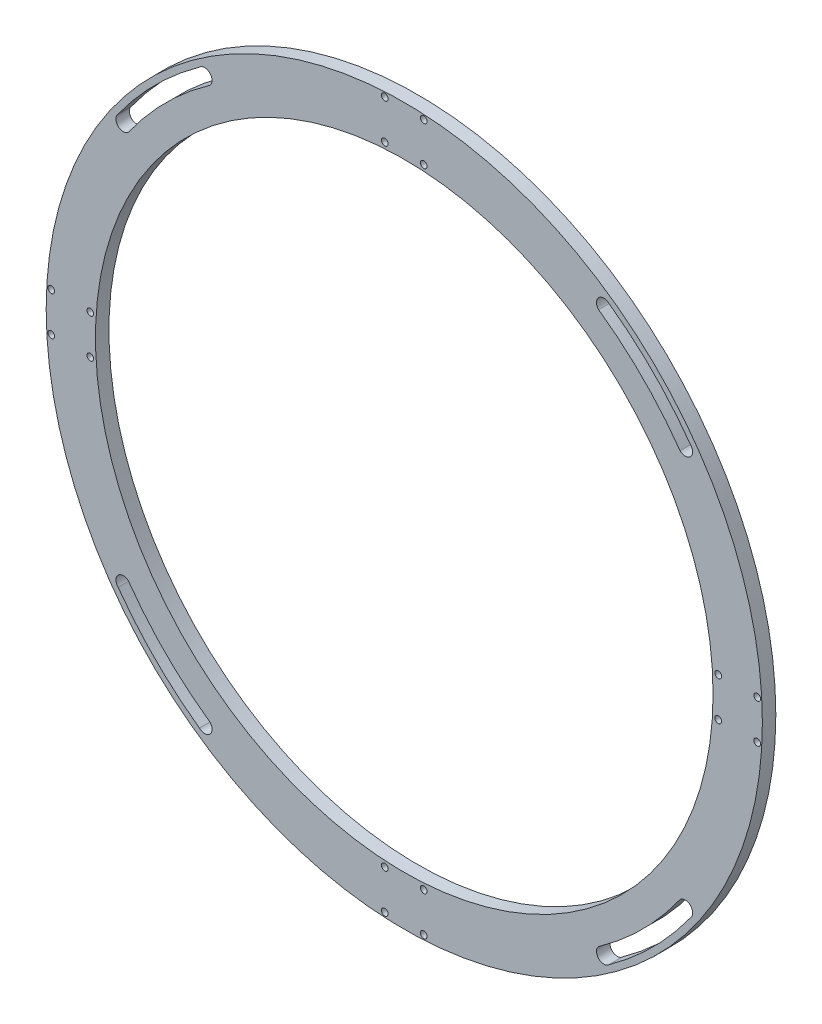
from build123d import *

# Parameters (mm, degrees)
SKETCH1_R           = 159.746139417
SKETCH1_R_2         = 1.5
SKETCH1_R_3         = 137.746139417
BOSS_EXTRUDE1_DEPTH = 6


with BuildPart() as part:
    # Sketch1 → Boss-Extrude1 (new body)
    with BuildSketch(Plane.XY):
        Circle(SKETCH1_R)
        with BuildLine():
            ThreePointArc((-91.383895087, -127.663556737), (-111.015764646, -111.015764646), (-127.663556737, -91.383895087))
            ThreePointArc((-127.663556737, -91.383895087), (-127.684062187, -86.718774861), (-123.01894196, -86.698269411))
            ThreePointArc((-123.01894196, -86.698269411), (-106.419570569, -106.419570569), (-86.698269411, -123.01894196))
            ThreePointArc((-86.698269411, -123.01894196), (-86.718774861, -127.684062187), (-91.383895087, -127.663556737))
        make_face(mode=Mode.SUBTRACT)
        with Locations((-8.7, -157.446139417)):
            Circle(SKETCH1_R_2, mode=Mode.SUBTRACT)
        with Locations((-8.7, -140.046139417)):
            Circle(SKETCH1_R_2, mode=Mode.SUBTRACT)
        with Locations((-157.446139417, -8.7)):
            Circle(SKETCH1_R_2, mode=Mode.SUBTRACT)
        with Locations((-140.046139417, -8.7)):
            Circle(SKETCH1_R_2, mode=Mode.SUBTRACT)
        with Locations((8.7, -157.446139417)):
            Circle(SKETCH1_R_2, mode=Mode.SUBTRACT)
        with Locations((8.7, -140.046139417)):
            Circle(SKETCH1_R_2, mode=Mode.SUBTRACT)
        with BuildLine():
            ThreePointArc((127.663556737, -91.383895087), (111.015764646, -111.015764646), (91.383895087, -127.663556737))
            ThreePointArc((91.383895087, -127.663556737), (86.718774861, -127.684062187), (86.698269411, -123.01894196))
            ThreePointArc((86.698269411, -123.01894196), (106.419570569, -106.419570569), (123.01894196, -86.698269411))
            ThreePointArc((123.01894196, -86.698269411), (127.684062187, -86.718774861), (127.663556737, -91.383895087))
        make_face(mode=Mode.SUBTRACT)
        with Locations((140.046139417, -8.7)):
            Circle(SKETCH1_R_2, mode=Mode.SUBTRACT)
        with Locations((157.446139417, -8.7)):
            Circle(SKETCH1_R_2, mode=Mode.SUBTRACT)
        with Locations((-157.446139417, 8.7)):
            Circle(SKETCH1_R_2, mode=Mode.SUBTRACT)
        with Locations((-140.046139417, 8.7)):
            Circle(SKETCH1_R_2, mode=Mode.SUBTRACT)
        with BuildLine():
            ThreePointArc((-127.663556737, 91.383895087), (-111.015764646, 111.015764646), (-91.383895087, 127.663556737))
            ThreePointArc((-91.383895087, 127.663556737), (-86.718774861, 127.684062187), (-86.698269411, 123.01894196))
            ThreePointArc((-86.698269411, 123.01894196), (-106.419570569, 106.419570569), (-123.01894196, 86.698269411))
            ThreePointArc((-123.01894196, 86.698269411), (-127.684062187, 86.718774861), (-127.663556737, 91.383895087))
        make_face(mode=Mode.SUBTRACT)
        with Locations((-8.7, 140.046139417)):
            Circle(SKETCH1_R_2, mode=Mode.SUBTRACT)
        with Locations((-8.7, 157.446139417)):
            Circle(SKETCH1_R_2, mode=Mode.SUBTRACT)
        Circle(SKETCH1_R_3, mode=Mode.SUBTRACT)
        with Locations((140.046139417, 8.7)):
            Circle(SKETCH1_R_2, mode=Mode.SUBTRACT)
        with Locations((157.446139417, 8.7)):
            Circle(SKETCH1_R_2, mode=Mode.SUBTRACT)
        with Locations((8.7, 140.046139417)):
            Circle(SKETCH1_R_2, mode=Mode.SUBTRACT)
        with Locations((8.7, 157.446139417)):
            Circle(SKETCH1_R_2, mode=Mode.SUBTRACT)
        with BuildLine():
            ThreePointArc((91.383895087, 127.663556737), (111.015764646, 111.015764646), (127.663556737, 91.383895087))
            ThreePointArc((127.663556737, 91.383895087), (127.684062187, 86.718774861), (123.01894196, 86.698269411))
            ThreePointArc((123.01894196, 86.698269411), (106.419570569, 106.419570569), (86.698269411, 123.01894196))
            ThreePointArc((86.698269411, 123.01894196), (86.718774861, 127.684062187), (91.383895087, 127.663556737))
        make_face(mode=Mode.SUBTRACT)
    extrude(amount=BOSS_EXTRUDE1_DEPTH)


solid = part.part
